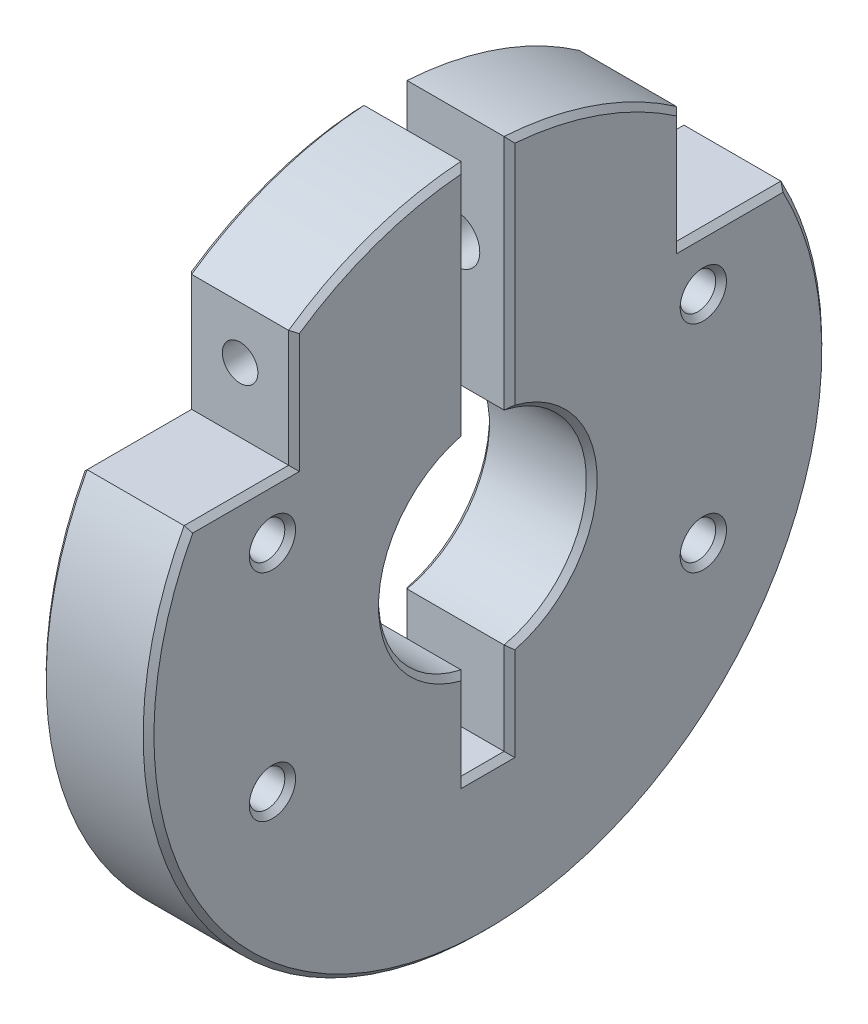
from build123d import *

# Parameters (mm, degrees)
BOSS_EXTRUDE1_DEPTH                                  = 5
HOLE_SIZE_BY_SOCKET_HEAD_CAP_SCREW_TYPE1_D           = 4.5
HOLE_SIZE_BY_SOCKET_HEAD_CAP_SCREW_TYPE1_DEPTH       = 16
HOLE_SIZE_BY_SOCKET_HEAD_CAP_SCREW_TYPE1_CBORE_D     = 8
HOLE_SIZE_BY_SOCKET_HEAD_CAP_SCREW_TYPE1_CBORE_DEPTH = 4.6
M4_TAPPED_HOLE1_D                                    = 3.3
M4_TAPPED_HOLE2_D                                    = 3.3
CHAMFER1_SIZE                                        = 0.5


with BuildPart() as part:
    # Sketch1 → Boss-Extrude1 (new, symmetric)
    with BuildSketch(Plane(origin=(0, 0, 0), x_dir=(0, 0, -1), z_dir=(1, 0, 0))):
        with BuildLine():
            Line((2, -9.440471387), (2, -18))
            Line((2, -18), (-2, -18))
            Line((-2, -18), (-2, -9.440471387))
            ThreePointArc((-2, -9.440471387), (-9.65, 0), (-2, 9.440471387))
            Line((-2, 9.440471387), (-2, 31.436443819))
            ThreePointArc((-2, 31.436443819), (-10.382706919, 29.739693963), (-18, 25.850531909))
            Line((-18, 25.850531909), (-18, 15))
            Line((-18, 15), (-27.699277969, 15))
            ThreePointArc((-27.699277969, 15), (0, -31.5), (27.699277969, 15))
            Line((27.699277969, 15), (18, 15))
            Line((18, 15), (18, 25.850531909))
            ThreePointArc((18, 25.850531909), (10.382706919, 29.739693963), (2, 31.436443819))
            Line((2, 31.436443819), (2, 9.440471387))
            ThreePointArc((2, 9.440471387), (9.65, 0), (2, -9.440471387))
        make_face()
    extrude(amount=BOSS_EXTRUDE1_DEPTH, both=True)

    # Hole size by socket head cap screw type1
    with Locations(Plane(origin=(0, 0, -18), x_dir=(-1, 0, 0), z_dir=(0, 0, -1))):
        with Locations((0, 21)):
            CounterBoreHole(HOLE_SIZE_BY_SOCKET_HEAD_CAP_SCREW_TYPE1_D / 2, HOLE_SIZE_BY_SOCKET_HEAD_CAP_SCREW_TYPE1_CBORE_D / 2, HOLE_SIZE_BY_SOCKET_HEAD_CAP_SCREW_TYPE1_CBORE_DEPTH, depth=HOLE_SIZE_BY_SOCKET_HEAD_CAP_SCREW_TYPE1_DEPTH)

    # M4 Tapped Hole1 (through all)
    with Locations(Plane(origin=(0, 0, 2), x_dir=(-1, 0, 0), z_dir=(0, 0, -1))):
        with Locations((0, 21)):
            Hole(M4_TAPPED_HOLE1_D / 2)

    # M4 Tapped Hole2 (through all)
    with Locations(Plane(origin=(5, 0, 0), x_dir=(0, 0, -1), z_dir=(1, 0, 0))):
        with Locations((20, 10), (20, -10), (-20, -10), (-20, 10)):
            Hole(M4_TAPPED_HOLE2_D / 2)

    # Chamfer1
    chamfer1_edges = [part.edges().sort_by_distance(p)[0] for p in [
        (5, 0, -9.65),
        (-5, 20.425265955, -18),
        (-5, 15, -22.849638984),
        (5, -13.720235693, -2),
        (-5, -31.5, 0),
        (-5, 15, 22.849638984),
        (-5, 20.425265955, 18),
        (-5, 29.739693963, 10.382706919),
        (-5, 20.438457603, 2),
        (-5, 0, 9.65),
        (-5, -13.720235693, 2),
        (5, -18, 0),
        (-5, -18, 0),
        (-5, -13.720235693, -2),
        (-5, 0, -9.65),
        (-5, 20.438457603, -2),
        (-5, 29.739693963, -10.382706919),
        (5, -13.720235693, 2),
        (5, 0, 9.65),
        (5, 20.438457603, 2),
        (5, 29.739693963, 10.382706919),
        (5, 20.425265955, 18),
        (5, 15, 22.849638984),
        (5, -31.5, 0),
        (5, 29.739693963, -10.382706919),
        (5, 15, -22.849638984),
        (5, 20.425265955, -18),
        (5, 10, 18.35),
        (-5, 10, 18.35),
        (5, -10, 18.35),
        (-5, -10, 18.35),
        (5, -10, -21.65),
        (-5, -10, -21.65),
        (5, 10, -21.65),
        (-5, 10, -21.65),
        (5, 20.438457603, -2),
    ]]
    chamfer(chamfer1_edges, length=CHAMFER1_SIZE)


solid = part.part
